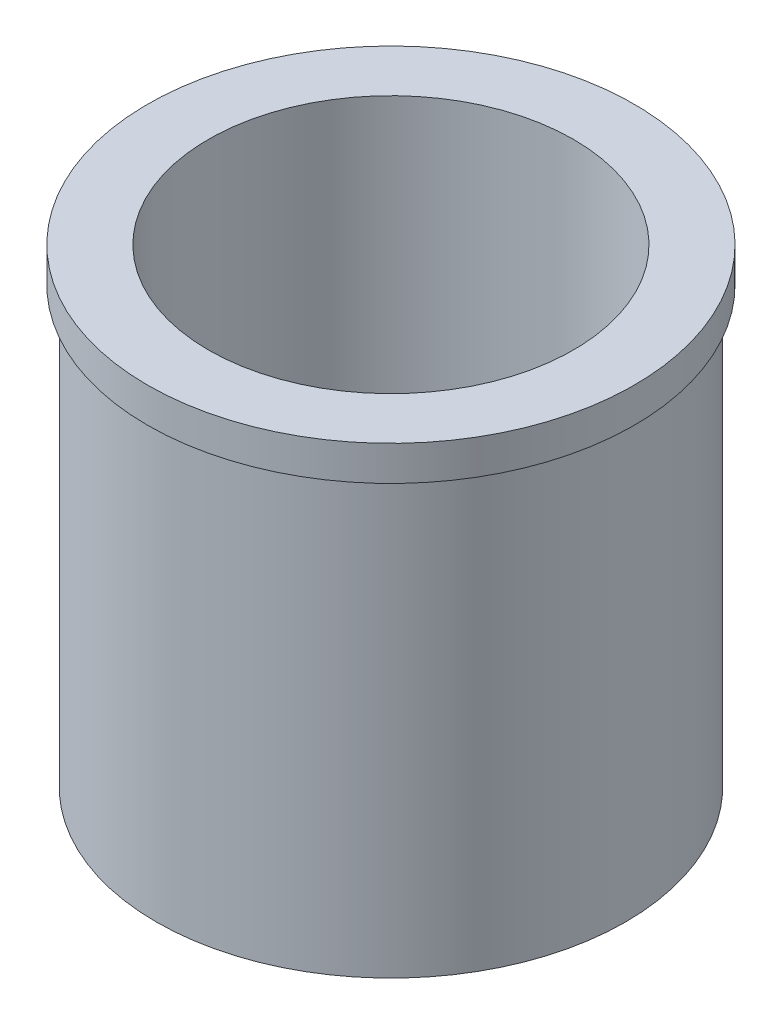
SolidWorks part; units mm, degrees
ref_plane "前视基准面" through (0, 0, 0) normal (0, 0, 1) x (1, 0, 0)
ref_plane "上视基准面" through (0, 0, 0) normal (0, 1, 0) x (1, 0, 0)
ref_plane "右视基准面" through (0, 0, 0) normal (1, 0, 0) x (0, 0, -1)
sketch "草图1" plane through (0, 0, 0) normal (0, 0, 1) x (1, 0, 0)
  line L0 (10.5, 0) -> (14, 0)
  line L1 (14, 0) -> (14, -2)
  line L2 (14, -2) -> (13.5, -2)
  line L3 (13.5, -2) -> (13.5, -27)
  line L4 (10.5, 0) -> (10.5, -27)
  line L5 (10.5, -27) -> (13.5, -27)
  line L6 (0, 4.077) -> (0, -7.3531) construction
  dimension "D1" = 14
  dimension "D2" = 10.5
  dimension "D3" = 2
  dimension "D4" = 13.5
  dimension "D5" = 25
revolve "旋转1" add sketch "草图1" angle 360 about L6
